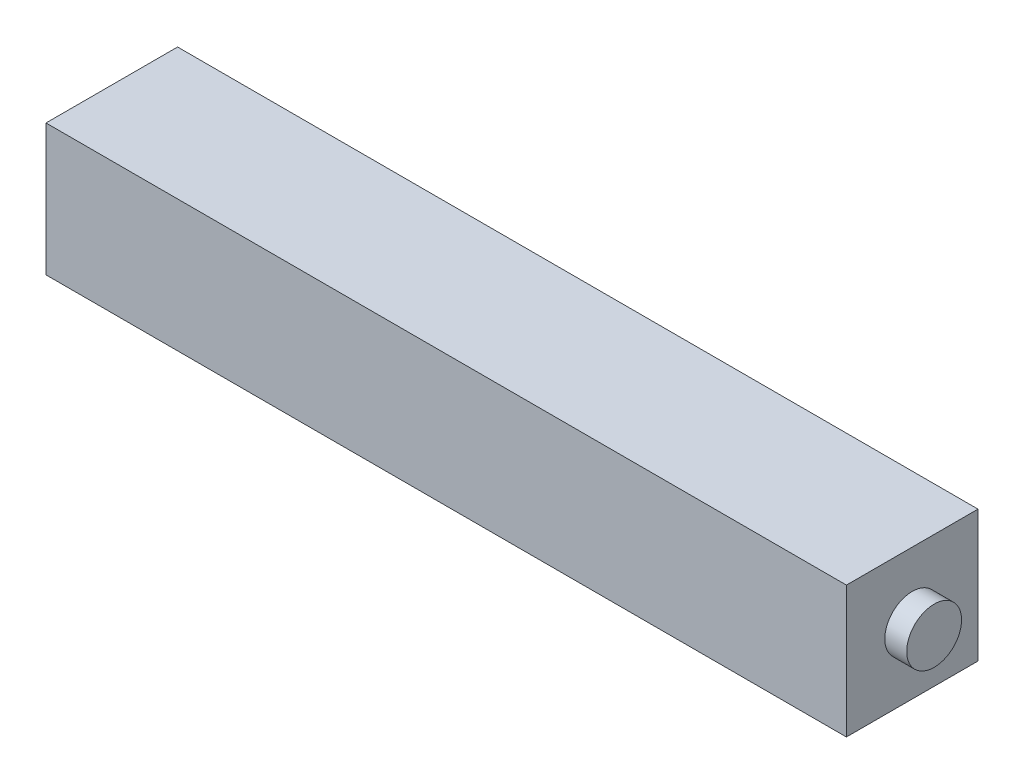
from build123d import *

# Parameters (mm, degrees)
SKETCH1_W           = 75
SKETCH1_H           = 12
BOSS_EXTRUDE1_DEPTH = 12
SKETCH2_OUTSIDE_W   = 29.38
SKETCH2_OUTSIDE_H   = 29.38
SKETCH2_OUTSIDE_R   = 2.5
CUT_EXTRUDE1_DEPTH  = 2


with BuildPart() as part:
    # Sketch1 → Boss-Extrude1 (new body)
    with BuildSketch(Plane.XY):
        Rectangle(SKETCH1_W, SKETCH1_H)
    extrude(amount=BOSS_EXTRUDE1_DEPTH)

    # Sketch2 outside → Cut-Extrude1 (cut)
    with BuildSketch(Plane(origin=(37.5, 0, 0), x_dir=(0, 0, -1), z_dir=(1, 0, 0))):
        with Locations((-6, 0)):
            Rectangle(SKETCH2_OUTSIDE_W, SKETCH2_OUTSIDE_H)
        with Locations((-6, 0)):
            Circle(SKETCH2_OUTSIDE_R, mode=Mode.SUBTRACT)
    extrude(amount=-CUT_EXTRUDE1_DEPTH, mode=Mode.SUBTRACT)


solid = part.part
